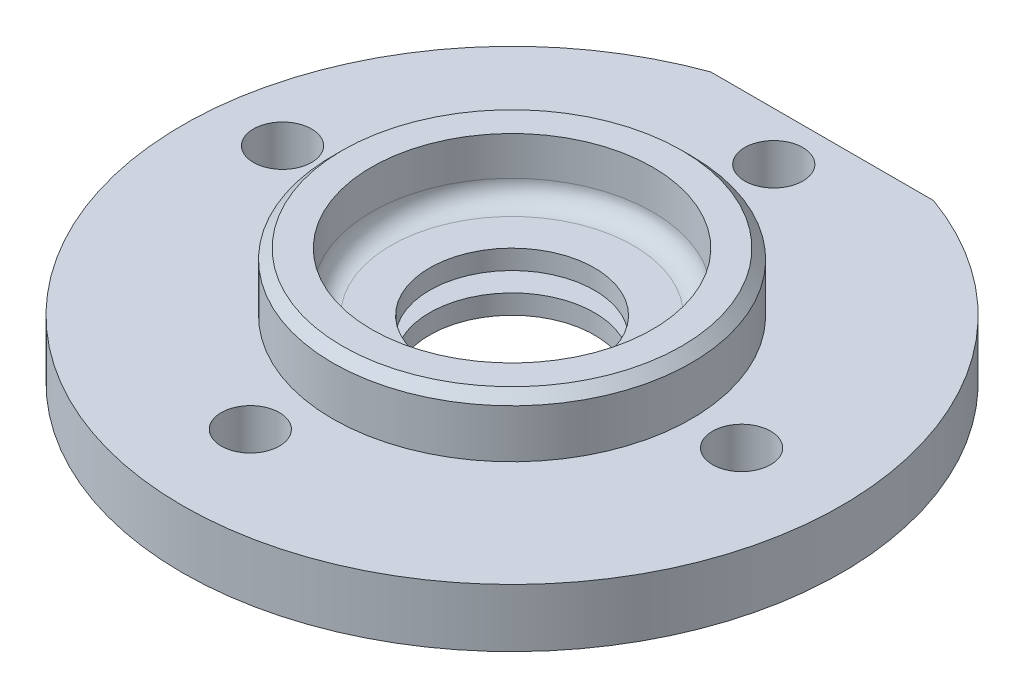
SolidWorks part; units mm, degrees
ref_plane "Front Plane" through (0, 0, 0) normal (0, 0, 1) x (1, 0, 0)
ref_plane "Top Plane" through (0, 0, 0) normal (0, 1, 0) x (1, 0, 0)
ref_plane "Right Plane" through (0, 0, 0) normal (1, 0, 0) x (0, 0, -1)
other "Configuration Table"
sketch "Sketch1" plane through (0, 0, 0) normal (0, 1, 0) x (1, 0, 0)
  circle A0 centre (0, 0) radius 34
  dimension "D1" = 68
extrude "Boss-Extrude1" add sketch "Sketch1" along normal blind 6
sketch "Sketch2" plane through (0, 6, 0) normal (0, 1, 0) x (1, 0, 0)
  circle A0 centre (0, 0) radius 18.5
  dimension "D1" = 37
extrude "Boss-Extrude2" add sketch "Sketch2" along normal blind 6
sketch "Sketch3" plane through (0, 12, 0) normal (0, 1, 0) x (1, 0, 0)
  circle A0 centre (0, 0) radius 14.5
  dimension "D1" = 29
extrude "Cut-Extrude1" cut sketch "Sketch3" against normal blind 6
sketch "Sketch4" plane through (0, 6, 0) normal (0, 1, 0) x (1, 0, 0)
  circle A0 centre (0, 0) radius 8.5
  dimension "D1" = 17
extrude "Cut-Extrude2" cut sketch "Sketch4" against normal blind 2
sketch "Sketch5" plane through (0, 4, 0) normal (0, 1, 0) x (1, 0, 0)
  circle A0 centre (0, 0) radius 12.5
  dimension "D1" = 25
extrude "Cut-Extrude3" cut sketch "Sketch5" against normal blind 2
sketch "Sketch6" plane through (0, 2, 0) normal (0, 1, 0) x (1, 0, 0)
  circle A0 centre (0, 0) radius 8.5
  dimension "D1" = 17
extrude "Cut-Extrude4" cut sketch "Sketch6" against normal blind 2
chamfer "Chamfer1" distance 1 angle 45 1 edges at (0, 12, 18.5)
fillet "Fillet1" radius 2 1 edges at (0, 6, 14.5)
sketch "Sketch7" plane through (0, 6, 0) normal (0, 1, 0) x (1, 0, 0)
  line L1 (-19.6234, 36) -> (19.6234, 36)
  line L2 (-19.6234, 36) -> (-19.6234, 32)
  line L3 (-19.6234, 32) -> (19.6234, 32)
  line L4 (19.6234, 36) -> (19.6234, 32)
  line L5 (-19.6234, 36) -> (19.6234, 32) construction
  line L6 (-19.6234, 32) -> (19.6234, 36) construction
  circle A0 centre (0, 0) radius 34 construction
  point P0 (0, 34)
  dimension "D1" = 32
extrude "Cut-Extrude5" cut sketch "Sketch7" against normal blind 23
sketch "Sketch8" plane through (0, 6, 0) normal (0, 1, 0) x (1, 0, 0)
  circle A0 centre (0, 0) radius 27 construction
  circle A1 centre (0, 27) radius 3
  circle A2 centre (23.68, 0) radius 3
  circle A3 centre (-3.32, -23.68) radius 3
  circle A4 centre (-27, 3.32) radius 3
  point P14 (-1.66, 1.66)
  dimension "D1" = 54
  dimension "D2" = 6
  dimension "D3" = 4
extrude "Cut-Extrude6" cut sketch "Sketch8" against normal blind 80
